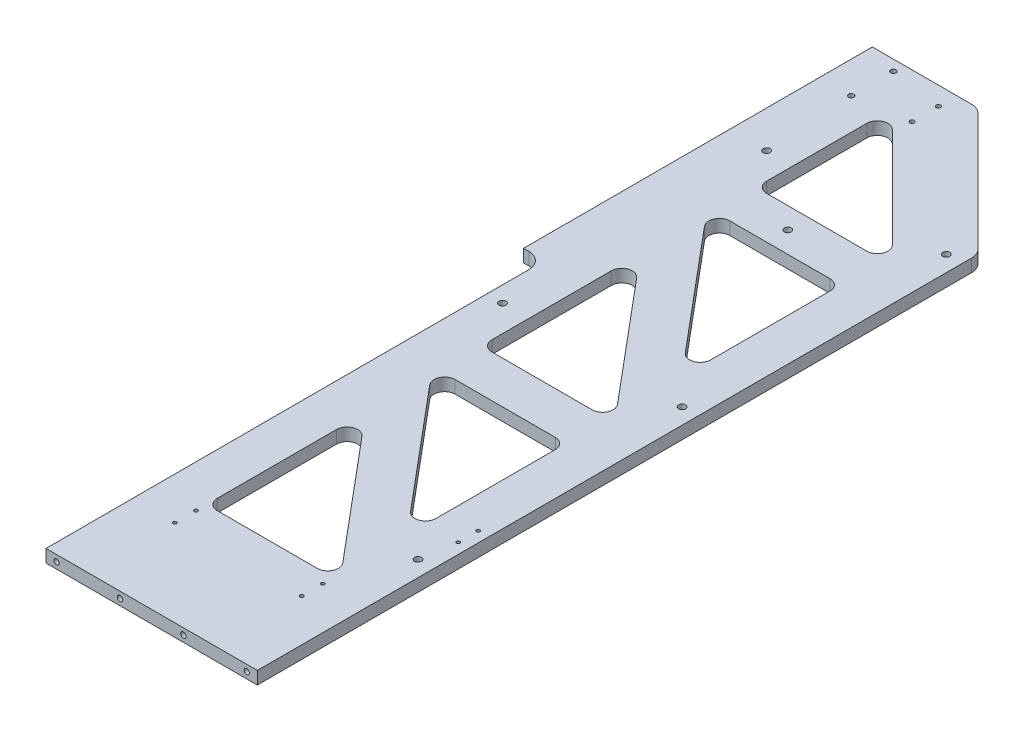
SolidWorks part; units mm, degrees
material "A6061"
ref_plane "前基準面" through (0, 0, 0) normal (0, 0, 1) x (1, 0, 0)
ref_plane "上基準面" through (0, 0, 0) normal (0, 1, 0) x (1, 0, 0)
ref_plane "右基準面" through (0, 0, 0) normal (1, 0, 0) x (0, 0, -1)
sketch "草图1" plane through (0, 0, 0) normal (0, 1, 0) x (1, 0, 0)
  line L1 (-110, -165) -> (110, -165)
  line L2 (-110, -165) -> (-110, 165)
  line L3 (-110, 165) -> (110, 165)
  line L4 (110, -165) -> (110, 165)
  line L5 (-110, -165) -> (110, 165) construction
  line L6 (-110, 165) -> (110, -165) construction
  point P0 (0, 0)
  dimension "D1" = 220
  dimension "D2" = 330
extrude "凸台-拉伸1" add sketch "草图1" along normal mid plane 12
sketch "草图2" plane through (0, 6, 0) normal (0, 1, 0) x (1, 0, 0)
  line L0 (110, 165) -> (-110, 165) construction
  line L1 (110, -165) -> (-90, -165)
  line L2 (110, -165) -> (110, -637)
  line L3 (110, -637) -> (-90, -637)
  line L4 (-90, -165) -> (-90, -637)
  dimension "D1" = 200
  dimension "D2" = 802
extrude "凸台-拉伸2" add sketch "草图2" against normal up to surface (12 mm away) up to face at (0, -6, 0)
chamfer "倒角1" distance 120 angle 45 1 edges at (110, 0, -165)
fillet "圆角2" radius 15 3 edges at (-10, 0, -165) (110, 0, -45)
sketch "草图7" plane through (0, 6, 0) normal (0, 1, 0) x (1, 0, 0)
  line L0 (-34.7477, -45) -> (60, -45)
  line L1 (70, -55) -> (70, -167.916)
  line L2 (52.3396, -174.3438) -> (-42.4082, -61.4279)
  line L3 (-32.3396, -135.6562) -> (62.4082, -248.5721)
  line L4 (54.7477, -265) -> (-40, -265)
  line L5 (105.6066, 49.3934) -> (-5.6066, 160.6066) construction
  line L6 (-50, -255) -> (-50, -142.084)
  line L7 (-16.2132, 165) -> (-110, 165) construction
  line L9 (110, -637) -> (110, 38.7868) construction
  line L10 (-90, -180) -> (-90, -637) construction
  line L13 (-34.7477, -305) -> (60, -305)
  line L14 (70, -315) -> (70, -427.916)
  line L15 (52.3396, -434.3438) -> (-42.4082, -321.4279)
  line L16 (-32.3396, -395.6562) -> (62.4082, -508.5721)
  line L17 (54.7477, -525) -> (-40, -525)
  line L18 (-50, -515) -> (-50, -402.084)
  line L20 (-50, 99.7477) -> (-50, 5)
  line L21 (-40, -5) -> (54.7477, -5)
  line L22 (61.8188, 12.0711) -> (-32.9289, 106.8188)
  line L25 (-50, -775) -> (-50, -662.084) [skipped]
  line L26 (-32.3396, -655.6562) -> (62.4082, -768.5721) [skipped]
  line L27 (54.7477, -785) -> (-40, -785) [skipped]
  line L28 (-34.7477, -565) -> (60, -565) [skipped]
  line L29 (70, -575) -> (70, -687.916) [skipped]
  line L30 (52.3396, -694.3438) -> (-42.4082, -581.4279) [skipped]
  arc A0 (62.4082, -248.5721) -> (54.7477, -265) centre (54.7477, -255) cw
  arc A1 (-32.3396, -135.6562) -> (-50, -142.084) centre (-40, -142.084) ccw
  arc A2 (-40, -265) -> (-50, -255) centre (-40, -255) cw
  arc A3 (60, -45) -> (70, -55) centre (60, -55) cw
  arc A4 (70, -167.916) -> (52.3396, -174.3438) centre (60, -167.916) cw
  arc A5 (-34.7477, -45) -> (-42.4082, -61.4279) centre (-34.7477, -55) ccw
  arc A6 (62.4082, -508.5721) -> (54.7477, -525) centre (54.7477, -515) cw
  arc A7 (-32.3396, -395.6562) -> (-50, -402.084) centre (-40, -402.084) ccw
  arc A8 (-40, -525) -> (-50, -515) centre (-40, -515) cw
  arc A9 (60, -305) -> (70, -315) centre (60, -315) cw
  arc A10 (70, -427.916) -> (52.3396, -434.3438) centre (60, -427.916) cw
  arc A11 (-34.7477, -305) -> (-42.4082, -321.4279) centre (-34.7477, -315) ccw
  arc A12 (-50, 99.7477) -> (-32.9289, 106.8188) centre (-40, 99.7477) cw
  arc A13 (54.7477, -5) -> (61.8188, 12.0711) centre (54.7477, 5) ccw
  arc A14 (-50, 5) -> (-40, -5) centre (-40, 5) ccw
  arc A21 (-32.3396, -655.6562) -> (-50, -662.084) centre (-40, -662.084) ccw [skipped]
  arc A22 (-40, -785) -> (-50, -775) centre (-40, -775) cw [skipped]
  arc A23 (62.4082, -768.5721) -> (54.7477, -785) centre (54.7477, -775) cw [skipped]
  arc A24 (60, -565) -> (70, -575) centre (60, -575) cw [skipped]
  arc A25 (70, -687.916) -> (52.3396, -694.3438) centre (60, -687.916) cw [skipped]
  arc A26 (-34.7477, -565) -> (-42.4082, -581.4279) centre (-34.7477, -575) ccw [skipped]
extrude "切除-拉伸3" cut sketch "草图7" against normal up to surface (12 mm away)
hole_wizard "M6 螺纹孔1" positions "草图11" profile "草图10" tap size "M6" standard "GB"
sketch "草图11" plane through (0, 0, 637) normal (0, 0, 1) x (1, 0, 0)
  line L0 (10, 6) -> (10, -6) construction
  line L1 (-90, 6) -> (110, 6) construction
  line L2 (-90, -6) -> (110, -6) construction
  line L4 (-90, 0) -> (-80, 0) construction
  line L5 (-90, -6) -> (-90, 6) construction
  point P0 (-80, 0)
  point P2 (-20, 0)
  point P13 (40, 0)
  point P14 (100, 0)
  dimension "D1" = 60
  dimension "D2" = 60
sketch "草图10" plane through (-80, 0, 637) normal (1, 0, 0) x (0, -1, 0)
  line L0 (0, 0) -> (0, 18.5022)
  line L1 (0, 18.5022) -> (2.5, 17)
  line L2 (2.5, 17) -> (2.5, 0)
  line L5 (2.5, 0) -> (0, 0)
  line L10 (0, 18.5022) -> (-2.5, 17) construction
  line L11 (0, -6.35) -> (0, 107.95) construction
  dimension "螺纹孔钻头直径" = 5
  dimension "螺纹孔钻头深度" = 17
  dimension "导头角度" = 118
cosmetic thread "孔螺蚊线9" parameters "D1"=12, "D2"=6
cosmetic thread "孔螺蚊线10" parameters "D1"=12, "D2"=6
cosmetic thread "孔螺蚊线11" parameters "D1"=12, "D2"=6
cosmetic thread "孔螺蚊线12" parameters "D1"=12, "D2"=6
hole_wizard "M6 螺纹孔2" positions "草图13" profile "草图12" tap size "M6" standard "GB"
sketch "草图13" plane through (-110, 0, 0) normal (-1, 0, 0) x (0, 0, 1)
  line L0 (0, 6) -> (0, -6) construction
  line L1 (-165, 6) -> (165, 6) construction
  line L2 (-165, -6) -> (165, -6) construction
  point P0 (-150, 0)
  point P23 (-90, 0)
  point P24 (-30, 0)
  point P25 (30, 0)
  point P26 (90, 0)
  point P27 (150, 0)
  dimension "D1" = 6
  dimension "D2" = 60
sketch "草图12" plane through (-110, 0, -150) normal (0, 1, 0) x (0, 0, 1)
  line L0 (0, 0) -> (0, 18.5022)
  line L1 (0, 18.5022) -> (2.5, 17)
  line L2 (2.5, 17) -> (2.5, 0)
  line L5 (2.5, 0) -> (0, 0)
  line L10 (0, 18.5022) -> (-2.5, 17) construction
  line L11 (0, -6.35) -> (0, 107.95) construction
  dimension "螺纹孔钻头直径" = 5
  dimension "螺纹孔钻头深度" = 17
  dimension "导头角度" = 118
cosmetic thread "孔螺蚊线5" parameters "D1"=12, "D2"=6
cosmetic thread "孔螺蚊线6" parameters "D1"=12, "D2"=6
cosmetic thread "孔螺蚊线7" parameters "D1"=12, "D2"=6
cosmetic thread "孔螺蚊线8" parameters "D1"=12, "D2"=6
cosmetic thread "孔螺蚊线17" parameters "D1"=12, "D2"=6
cosmetic thread "孔螺蚊线18" parameters "D1"=12, "D2"=6
hole_wizard "M6 间隙孔1" positions "草图14" profile "草图15" hole size "M6" standard "GB"
sketch "草图14" plane through (0, 6, 0) normal (0, 1, 0) x (1, 0, 0)
  line L0 (10, -637) -> (10, -112.3238) construction
  line L1 (-90, -637) -> (110, -637) construction
  line L3 (110, -637) -> (110, 38.7868) construction
  point P0 (95, 30)
  point P7 (-75, 30)
  point P8 (-75, -220)
  point P10 (95, -220)
  point P11 (95, -470)
  point P22 (-75, -470) [skipped]
  dimension "D3" = 15
  dimension "D4" = 250
  dimension "D5" = 167
  dimension "D1" = 2
  dimension "D2" = 3
sketch "草图15" plane through (95, 6, -30) normal (1, 0, 0) x (0, 0, 1)
  line L0 (0, 0) -> (0, 12)
  line L1 (0, 12) -> (3.3, 12)
  line L2 (3.3, 12) -> (3.3, 0)
  line L5 (3.3, 0) -> (0, 0)
  line L11 (0, -6.35) -> (0, 107.95) construction
  dimension "通孔孔直径" = 6.6
  dimension "通孔孔深度" = 12
hole_wizard "M6 间隙孔2" positions "草图16" profile "草图17" hole size "M6" standard "GB" end condition through all
sketch "草图16" plane through (0, 6, 0) normal (0, 1, 0) x (1, 0, 0)
  line L0 (0, -5) -> (0, -45) construction
  line L1 (-40, -5) -> (54.7477, -5) construction
  line L2 (60, -45) -> (-34.7477, -45) construction
  point P0 (0, -25)
sketch "草图17" plane through (0, 6, 25) normal (1, 0, 0) x (0, 0, 1)
  line L0 (0, 0) -> (0, 12)
  line L1 (0, 12) -> (3.3, 12)
  line L2 (3.3, 12) -> (3.3, 0)
  line L5 (3.3, 0) -> (0, 0)
  line L11 (0, -6.35) -> (0, 107.95) construction
  dimension "通孔孔直径" = 6.6
  dimension "通孔孔深度" = 12
hole_wizard "M6 螺纹孔3" positions "草图18" profile "草图19" tap size "M6" standard "GB" end condition through all
sketch "草图18" plane through (0, 6, 0) normal (0, 1, 0) x (1, 0, 0)
  line L0 (-16.2132, 165) -> (-110, 165) construction
  line L1 (-110, 165) -> (-110, -165) construction
  point P0 (-80, 155)
  point P2 (-80, 115)
  dimension "D1" = 40
  dimension "D2" = 10
  dimension "D3" = 30
sketch "草图19" plane through (-80, 6, -155) normal (1, 0, 0) x (0, 0, 1)
  line L0 (0, 0) -> (0, 12)
  line L1 (0, 12) -> (2.5, 12)
  line L2 (2.5, 12) -> (2.5, 0)
  line L5 (2.5, 0) -> (0, 0)
  line L11 (0, -6.35) -> (0, 107.95) construction
  dimension "通孔螺纹孔钻头直径" = 5
  dimension "通孔螺纹孔钻头深度" = 12
cosmetic thread "孔螺蚊线13" parameters "D2"=6
cosmetic thread "孔螺蚊线14" parameters "D2"=6
hole_wizard "M5 螺纹孔1" positions "草图20" profile "草图21" tap size "M5" standard "GB" end condition through all
sketch "草图20" plane through (0, 6, 0) normal (0, 1, 0) x (1, 0, 0)
  line L0 (-16.2132, 165) -> (-110, 165) construction
  line L1 (-110, 165) -> (-110, -165) construction
  point P0 (-30, 147.5)
  point P2 (-30, 122.5)
  dimension "D1" = 25
  dimension "D2" = 17.5
  dimension "D3" = 80
sketch "草图21" plane through (-30, 6, -147.5) normal (1, 0, 0) x (0, 0, 1)
  line L0 (0, 0) -> (0, 12)
  line L1 (0, 12) -> (2.1, 12)
  line L2 (2.1, 12) -> (2.1, 0)
  line L5 (2.1, 0) -> (0, 0)
  line L11 (0, -6.35) -> (0, 107.95) construction
  dimension "通孔螺纹孔钻头直径" = 4.2
  dimension "通孔螺纹孔钻头深度" = 12
cosmetic thread "孔螺蚊线15" parameters "D2"=5
cosmetic thread "孔螺蚊线16" parameters "D2"=5
hole_wizard "M4 螺纹孔1" positions "草图22" profile "草图23" tap size "M4" standard "GB" end condition through all
sketch "草图22" plane through (0, 6, 0) normal (0, 1, 0) x (1, 0, 0)
  line L0 (110, -637) -> (110, 38.7868) construction
  line L1 (-90, -637) -> (110, -637) construction
  point P0 (100, -418)
  point P2 (100, -437)
  dimension "D1" = 19
  dimension "D2" = 10
  dimension "D3" = 200
sketch "草图23" plane through (100, 6, 418) normal (1, 0, 0) x (0, 0, 1)
  line L0 (0, 0) -> (0, 12)
  line L1 (0, 12) -> (1.65, 12)
  line L2 (1.65, 12) -> (1.65, 0)
  line L5 (1.65, 0) -> (0, 0)
  line L11 (0, -6.35) -> (0, 107.95) construction
  dimension "通孔螺纹孔钻头直径" = 3.3
  dimension "通孔螺纹孔钻头深度" = 12
cosmetic thread "孔螺蚊线19" parameters "D2"=4
cosmetic thread "孔螺蚊线20" parameters "D2"=4
hole_wizard "M4 螺纹孔2" positions "草图24" profile "草图25" tap size "M4" standard "GB" end condition through all
sketch "草图24" plane through (0, -6, 0) normal (0, -1, 0) x (-1, 0, 0)
  line L1 (-10, -637) -> (-10, -525) construction
  line L2 (90, -637) -> (-110, -637) construction
  line L3 (40, -525) -> (-54.7477, -525) construction
  line L5 (-10, -545) -> (21.7845, -545) construction
  line L7 (21.7845, -525) -> (21.7845, -565) construction
  point P0 (-70, -535)
  point P2 (50, -555)
  point P5 (-70, -555)
  point P7 (50, -535)
  dimension "D1" = 120
  dimension "D2" = 20
  dimension "D3" = 10
sketch "草图25" plane through (70, -6, 535) normal (1, 0, 0) x (0, 0, -1)
  line L0 (0, 0) -> (0, 12)
  line L1 (0, 12) -> (1.65, 12)
  line L2 (1.65, 12) -> (1.65, 0)
  line L5 (1.65, 0) -> (0, 0)
  line L11 (0, -6.35) -> (0, 107.95) construction
  dimension "通孔螺纹孔钻头直径" = 3.3
  dimension "通孔螺纹孔钻头深度" = 12
cosmetic thread "孔螺蚊线21" parameters "D2"=4
cosmetic thread "孔螺蚊线22" parameters "D2"=4
cosmetic thread "孔螺蚊线23" parameters "D2"=4
cosmetic thread "孔螺蚊线24" parameters "D2"=4
equation "\"D3@草图7\"=\"D2@草图7\""
